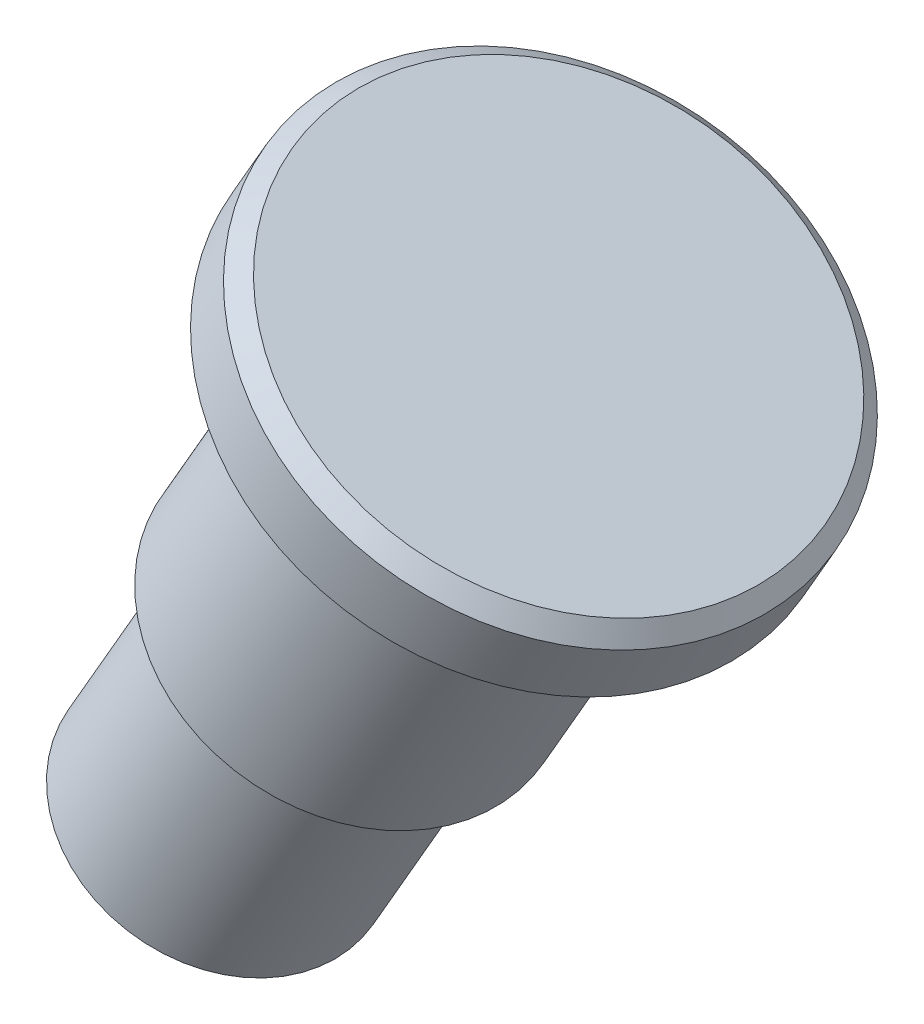
from build123d import *

# Parameters (mm, degrees)
CHAMFER1_SIZE = 0.5


with BuildPart() as part:
    # Sketch1 → Revolve1 (revolve)
    with BuildSketch(Plane.XY, mode=Mode.PRIVATE) as revolve1_sk:
        Polygon((-80.994872981, 46.440861912), (-78.829809472, 45.190861912), (-77.329809472, 47.788938123), (-83.825, 51.538938123), (-94.325, 33.352404644), (-90.860898385, 31.352404644), (-86.860898385, 38.280607874), (-85.994872981, 37.780607874), align=None)
    revolve(revolve1_sk.sketch.rotate(Axis((-83.825, 51.538938123, 0), (-0.499999999999998, -0.8660254037844399, 0)), 180), axis=Axis((-83.825, 51.538938123, 0), (-0.499999999999998, -0.8660254037844399, 0)))

    # Chamfer1
    chamfer1_edges = [part.edges().sort_by_distance(p)[0] for p in [
        (-85.994872981, 37.780607874, 0),
        (-90.860898385, 31.352404644, 0),
        (-77.329809472, 47.788938123, 0),
        (-78.829809472, 45.190861912, 0),
    ]]
    chamfer(chamfer1_edges, length=CHAMFER1_SIZE)


solid = part.part
